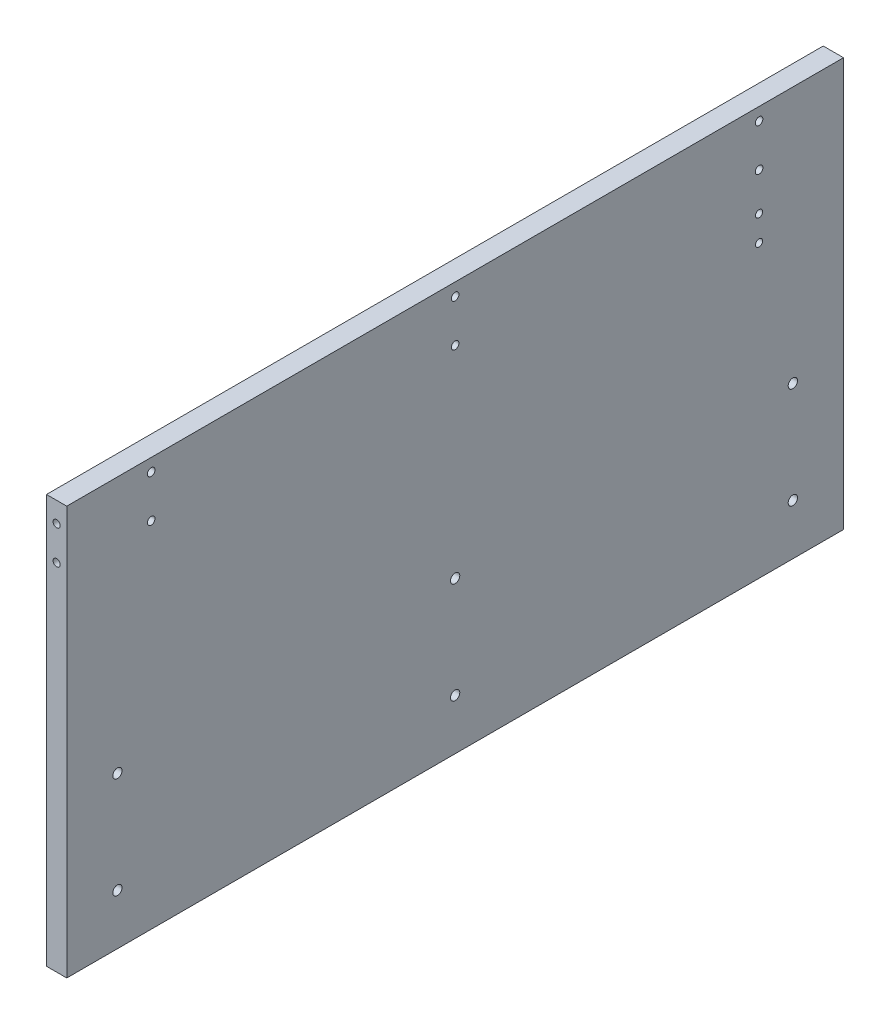
from build123d import *

# Parameters (mm, degrees)
SKETCH_1_W                  = 12
SKETCH_1_H                  = 242
EXTRUDE_1_DEPTH             = 230
HOLE_WIZARD_M5_1_D          = 4.2
HOLE_WIZARD_M5_1_DEPTH      = 14
HOLE_WIZARD_M5_1_TIP        = 1.2618073
HOLE_WIZARD_1_D             = 5.5
HOLE_WIZARD_1_DEPTH         = 14
HOLE_WIZARD_1_CBORE_D       = 10
HOLE_WIZARD_1_CBORE_DEPTH   = 5.7
HOLE_WIZARD_1_TIP           = 1.652366702
HOLE_WIZARD_2_D             = 4.5
HOLE_WIZARD_2_DEPTH         = 14
HOLE_WIZARD_2_CBORE_D       = 8
HOLE_WIZARD_2_CBORE_DEPTH   = 4.6
HOLE_WIZARD_2_TIP           = 1.351936393
HOLE_WIZARD_M5_2_AT_2_COUNT = 2
HOLE_WIZARD_M5_2_AT_2_PITCH = 20
HOLE_WIZARD_M5_3_D          = 4.2
HOLE_WIZARD_M5_3_DEPTH      = 14
HOLE_WIZARD_M5_3_TIP        = 1.2618073


with BuildPart() as part:
    # 草图1 → 凸台-拉伸1 (new, symmetric)
    with BuildSketch(Plane.XY):
        Rectangle(SKETCH_1_W, SKETCH_1_H)
    extrude(amount=EXTRUDE_1_DEPTH, both=True)

    # M5 螺纹孔1
    with Locations(Plane.XZ.offset(121)):
        with Locations((0, 200), (0, 0), (0, -200)):
            Hole(HOLE_WIZARD_M5_1_D / 2, depth=HOLE_WIZARD_M5_1_DEPTH)
            with Locations((0, 0, -(HOLE_WIZARD_M5_1_DEPTH + HOLE_WIZARD_M5_1_TIP / 2))):  # 118° drill point
                Cone(0, HOLE_WIZARD_M5_1_D / 2, HOLE_WIZARD_M5_1_TIP, mode=Mode.SUBTRACT)

    # 打孔尺寸(%根据)内六角圆柱头螺钉的类型1
    with Locations(Plane.ZY.offset(6)):
        with Locations((200, -31), (200, -91), (0, -31), (0, -91), (-200, -31), (-200, -91)):
            CounterBoreHole(HOLE_WIZARD_1_D / 2, HOLE_WIZARD_1_CBORE_D / 2, HOLE_WIZARD_1_CBORE_DEPTH, depth=HOLE_WIZARD_1_DEPTH)
            with Locations((0, 0, -(HOLE_WIZARD_1_DEPTH + HOLE_WIZARD_1_TIP / 2))):  # 118° drill point
                Cone(0, HOLE_WIZARD_1_D / 2, HOLE_WIZARD_1_TIP, mode=Mode.SUBTRACT)

    # 打孔尺寸(%根据)内六角圆柱头螺钉的类型2
    with Locations(Plane(origin=(-6, 0, 0), x_dir=(0, 0, -1), z_dir=(-1, 0, 0))):
        with Locations((180, -113.5), (180, -88.5), (0, -113.5), (0, -88.5), (-180, -113.5), (-180, -88.5)):
            CounterBoreHole(HOLE_WIZARD_2_D / 2, HOLE_WIZARD_2_CBORE_D / 2, HOLE_WIZARD_2_CBORE_DEPTH, depth=HOLE_WIZARD_2_DEPTH)
            with Locations((0, 0, -(HOLE_WIZARD_2_DEPTH + HOLE_WIZARD_2_TIP / 2))):  # 118° drill point
                Cone(0, HOLE_WIZARD_2_D / 2, HOLE_WIZARD_2_TIP, mode=Mode.SUBTRACT)

    # 草图8 → M5 螺纹孔2 (revolve, cut)
    with BuildSketch(Plane(origin=(0, 109, -230), x_dir=(0, 1, 0), z_dir=(1, 0, 0))):
        Polygon((0, 0), (0, 15.2618073), (2.1, 14), (2.1, 0), align=None)
    hole_wizard_m5_2 = revolve(axis=Axis((0, 109, -236.35), (0, 0, 1)), mode=Mode.SUBTRACT)

    # M5 螺纹孔2 at 2: M5 螺纹孔2 ×2
    with Locations(*[(0, -i * HOLE_WIZARD_M5_2_AT_2_PITCH, 0) for i in range(1, HOLE_WIZARD_M5_2_AT_2_COUNT)]):
        add(hole_wizard_m5_2, mode=Mode.SUBTRACT)

    # 镜向1: M5 螺纹孔2 across plane
    add(hole_wizard_m5_2.mirror(Plane.XY), mode=Mode.SUBTRACT)

    # 镜向1 copy 1 sketch → 镜向1 copy 1 (revolve, cut)
    with BuildSketch(Plane(origin=(0, 89, 230), x_dir=(0, 1, 0), z_dir=(1, 0, 0))):
        Polygon((0, 0), (0, -15.2618073), (2.1, -14), (2.1, 0), align=None)
    revolve(axis=Axis((0, 89, 236.35), (0, 0, 1)), mode=Mode.SUBTRACT)

    # M5 螺纹孔3
    with Locations(Plane(origin=(6, 0, 0), x_dir=(0, 0, -1), z_dir=(1, 0, 0))):
        with Locations((180, 66), (180, 51)):
            Hole(HOLE_WIZARD_M5_3_D / 2, depth=HOLE_WIZARD_M5_3_DEPTH)
            with Locations((0, 0, -(HOLE_WIZARD_M5_3_DEPTH + HOLE_WIZARD_M5_3_TIP / 2))):  # 118° drill point
                Cone(0, HOLE_WIZARD_M5_3_D / 2, HOLE_WIZARD_M5_3_TIP, mode=Mode.SUBTRACT)


solid = part.part
